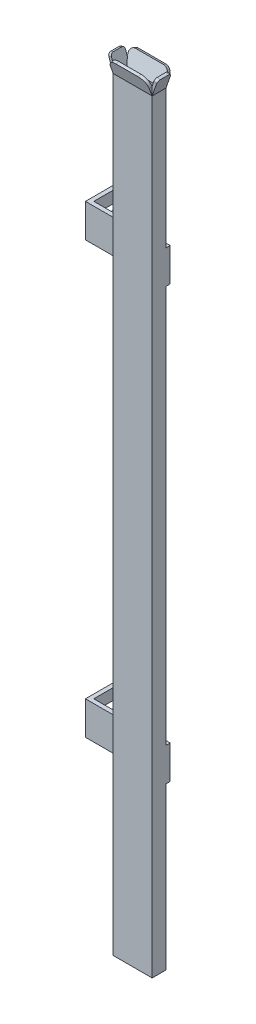
from build123d import *

# Parameters (mm, degrees)
SKETCH1_W           = 14
SKETCH1_H           = 5
SKETCH1_W_2         = 12
SKETCH1_H_2         = 3
BOSS_EXTRUDE1_DEPTH = 275
SKETCH2_W           = 29
SKETCH2_H           = 12
BOSS_EXTRUDE2_DEPTH = 1.5
SKETCH3_W           = 15
SKETCH3_H           = 12
BOSS_EXTRUDE3_DEPTH = 1.5
LPATTERN1_COUNT     = 2
LPATTERN1_PITCH     = 155
CHAMFER1_SIZE       = 1
CUT_EXTRUDE1_DEPTH  = 10
BOSS_EXTRUDE4_REACH = 279.078
FILLET1_R           = 3
BOSS_EXTRUDE5_REACH = 283.899
FILLET2_R           = 1
FILLET3_R           = 2


with BuildPart() as part:
    # Sketch1 → Boss-Extrude1 (new body)
    with BuildSketch(Plane(origin=(0, 0, 0), x_dir=(1, 0, 0), z_dir=(0, 1, 0))):
        Rectangle(SKETCH1_W, SKETCH1_H)
        Rectangle(SKETCH1_W_2, SKETCH1_H_2, mode=Mode.SUBTRACT)
    extrude(amount=BOSS_EXTRUDE1_DEPTH)

    # Sketch2 → Boss-Extrude2 (add)
    with BuildSketch(Plane(origin=(0, 0, -2.5), x_dir=(-1, 0, 0), z_dir=(0, 0, -1))):
        with Locations((7.5, 219)):
            Rectangle(SKETCH2_W, SKETCH2_H)
    boss_extrude2 = extrude(amount=BOSS_EXTRUDE2_DEPTH)

    # Sketch3 → Boss-Extrude3 (add)
    with BuildSketch(Plane.ZY.offset(22)):
        with Locations((-10, 219)):
            Rectangle(SKETCH3_W, SKETCH3_H)
    boss_extrude3 = extrude(amount=-BOSS_EXTRUDE3_DEPTH)

    # LPattern1: Boss-Extrude2, Boss-Extrude3 ×2
    with Locations(*[(0, -i * LPATTERN1_PITCH, 0) for i in range(1, LPATTERN1_COUNT)]):
        add(boss_extrude2)
        add(boss_extrude3)

    # Chamfer1
    chamfer1_edges = [part.edges().sort_by_distance(p)[0] for p in [
        (-21.25, 213, -17.5),
        (-21.25, 225, -17.5),
        (-21.25, 58, -17.5),
        (-21.25, 70, -17.5),
    ]]
    chamfer(chamfer1_edges, length=CHAMFER1_SIZE)

    # Sketch4 → Cut-Extrude1 (cut)
    with BuildSketch(Plane(origin=(-20.5, 0, 0), x_dir=(0, 0, -1), z_dir=(1, 0, 0))):
        with BuildLine():
            Line((8, 66), (14, 66))
            ThreePointArc((14, 66), (16, 64), (14, 62))
            Line((14, 62), (8, 62))
            ThreePointArc((8, 62), (6, 64), (8, 66))
        make_face()
        with BuildLine():
            Line((14, 217.25), (8, 217.25))
            ThreePointArc((8, 217.25), (6.25, 219), (8, 220.75))
            Line((8, 220.75), (14, 220.75))
            ThreePointArc((14, 220.75), (15.75, 219), (14, 217.25))
        make_face()
    extrude(amount=-CUT_EXTRUDE1_DEPTH, mode=Mode.SUBTRACT)

    # Boss-Extrude4: up to this face of the body (flat: up to its plane)
    boss_extrude4_end = Plane(part.part.faces().sort_by_distance((-7, 137.5, 0))[0])
    # Sketch5 → Boss-Extrude4 (add, up to the picked face)
    with BuildSketch(Plane(origin=(7, 0, 0), x_dir=(0, 0, -1), z_dir=(1, 0, 0)), mode=Mode.PRIVATE) as boss_extrude4_sk1:
        Polygon((-1.5, 275), (-3.55212086, 280.638155725), (-4.491813481, 280.296135581), (-1.5, 272.0761956), align=None)
    boss_extrude4_tool1 = split(extrude(boss_extrude4_sk1.sketch, amount=-BOSS_EXTRUDE4_REACH, mode=Mode.PRIVATE), bisect_by=boss_extrude4_end, keep=Keep.BOTH, mode=Mode.PRIVATE)
    boss_extrude4 = boss_extrude4_tool1.solids().sort_by(Axis((7, 276.951919, 2.775572), (-1, 0, 0)))[0]
    add(boss_extrude4)

    # Fillet1
    fillet1_edges = [part.edges().sort_by_distance(p)[0] for p in [
        (7, 280.467145653, 4.02196717),
        (-7, 280.467145653, 4.02196717),
    ]]
    fillet(fillet1_edges, radius=FILLET1_R)

    # Boss-Extrude5: up to this face of the body (flat: up to its plane)
    boss_extrude5_end = Plane(part.part.faces().sort_by_distance((0, 137.41183651, 2.5))[0])
    # Sketch6 → Boss-Extrude5 (add, up to the picked face)
    with BuildSketch(Plane(origin=(0, 0, -2.5), x_dir=(-1, 0, 0), z_dir=(0, 0, -1)), mode=Mode.PRIVATE) as boss_extrude5_sk1:
        Polygon((-6, 275), (-7.953408927, 280.673111454), (-8.898927502, 280.347543299), (-6, 271.928446513), align=None)
    boss_extrude5_tool1 = split(extrude(boss_extrude5_sk1.sketch, amount=-BOSS_EXTRUDE5_REACH, mode=Mode.PRIVATE), bisect_by=boss_extrude5_end, keep=Keep.BOTH, mode=Mode.PRIVATE)
    # Sketch6 → Boss-Extrude5 (add, up to the picked face)
    with BuildSketch(Plane(origin=(0, 0, -2.5), x_dir=(-1, 0, 0), z_dir=(0, 0, -1)), mode=Mode.PRIVATE) as boss_extrude5_sk2:
        Polygon((6, 275), (6, 271.928446513), (8.898927502, 280.347543299), (7.953408927, 280.673111454), align=None)
    boss_extrude5_tool2 = split(extrude(boss_extrude5_sk2.sketch, amount=-BOSS_EXTRUDE5_REACH, mode=Mode.PRIVATE), bisect_by=boss_extrude5_end, keep=Keep.BOTH, mode=Mode.PRIVATE)
    add(boss_extrude5_tool1.solids().sort_by(Axis((7.228438, 276.932112, -2.5), (0, 0, 1)))[0])
    add(boss_extrude5_tool2.solids().sort_by(Axis((-7.228438, 276.932112, -2.5), (0, 0, 1)))[0])

    # Fillet2
    fillet2_edges = [part.edges().sort_by_distance(p)[0] for p in [
        (8.426168215, 280.510327376, 2.5),
        (8.426168215, 280.510327376, -2.5),
        (-8.426168215, 280.510327376, 2.5),
        (-8.426168215, 280.510327376, -2.5),
    ]]
    fillet(fillet2_edges, radius=FILLET2_R)

    # Mirror1: Boss-Extrude4 across plane
    add(boss_extrude4.mirror(Plane.XY))

    # Fillet3
    fillet3_edges = [part.edges().sort_by_distance(p)[0] for p in [
        (-7, 280.467145653, -4.02196717),
        (7, 280.467145653, -4.02196717),
    ]]
    fillet(fillet3_edges, radius=FILLET3_R)


solid = part.part
